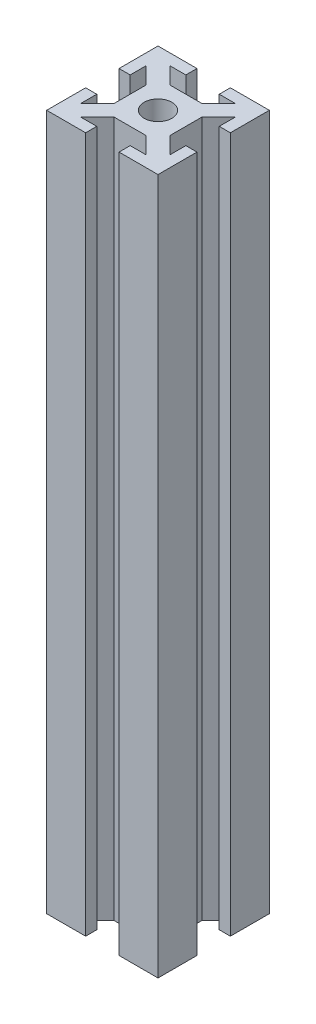
SolidWorks part; units mm, degrees
ref_plane "Front Plane" through (0, 0, 0) normal (0, 0, 1) x (1, 0, 0)
ref_plane "Top Plane" through (0, 0, 0) normal (0, 1, 0) x (1, 0, 0)
ref_plane "Right Plane" through (0, 0, 0) normal (1, 0, 0) x (0, 0, -1)
other "Configuration Table"
sketch "Sketch1" plane through (0, 0, 0) normal (0, 1, 0) x (1, 0, 0)
  line L0 (-6, 20) -> (-6, 16)
  line L5 (-20, 20) -> (-6, 20)
  line L6 (-20, 20) -> (-20, 6)
  line L7 (-20, -20) -> (-6, -20)
  line L8 (20, 20) -> (20, 6)
  line L9 (-20, 20) -> (20, -20) construction
  line L10 (-20, -20) -> (20, 20) construction
  line L11 (-6, 16) -> (-11.7574, 16)
  line L12 (-11.7574, 16) -> (-5.7574, 10)
  line L13 (5.7574, 10) -> (11.7574, 16)
  line L14 (11.7574, 16) -> (6, 16)
  line L15 (6, 16) -> (6, 20)
  line L16 (20, 6) -> (16, 6)
  line L17 (16, 6) -> (16, 11.7574)
  line L18 (16, 11.7574) -> (10, 5.7574)
  line L19 (10, -5.7574) -> (16, -11.7574)
  line L20 (16, -11.7574) -> (16, -6)
  line L21 (16, -6) -> (20, -6)
  line L22 (6, -20) -> (6, -16)
  line L23 (6, -16) -> (11.7574, -16)
  line L24 (11.7574, -16) -> (5.7574, -10)
  line L25 (-5.7574, -10) -> (-11.7574, -16)
  line L26 (-11.7574, -16) -> (-6, -16)
  line L27 (-6, -16) -> (-6, -20)
  line L28 (-20, -6) -> (-16, -6)
  line L29 (-16, -6) -> (-16, -11.7574)
  line L30 (-16, -11.7574) -> (-10, -5.7574)
  line L31 (-10, 5.7574) -> (-16, 11.7574)
  line L32 (-16, 11.7574) -> (-16, 6)
  line L33 (-16, 6) -> (-20, 6)
  line L34 (6, 20) -> (20, 20)
  line L35 (-20, -6) -> (-20, -20)
  line L36 (20, -6) -> (20, -20)
  line L37 (6, -20) -> (20, -20)
  line L39 (-5.7574, -10) -> (5.7574, -10)
  line L40 (-10, -5.7574) -> (-10, 5.7574)
  line L41 (-5.7574, 10) -> (5.7574, 10)
  line L42 (10, -5.7574) -> (10, 5.7574)
  line L43 (-10, -10) -> (10, 10) construction
  line L44 (-10, 10) -> (10, -10) construction
  circle A0 centre (0, 0) radius 5
  point P0 (0, 0)
  point P5 (0, 0)
  point P37 (0, 0)
  dimension "D10" = 10
  dimension "D1" = 40
  dimension "D2" = 4
  dimension "D3" = 4
  dimension "D4" = 14
  dimension "D5" = 14
  dimension "D6" = 3
  dimension "D7" = 3
  dimension "D8" = 4
  dimension "D9" = 20
extrude "Boss-Extrude1" add sketch "Sketch1" along normal blind 250
